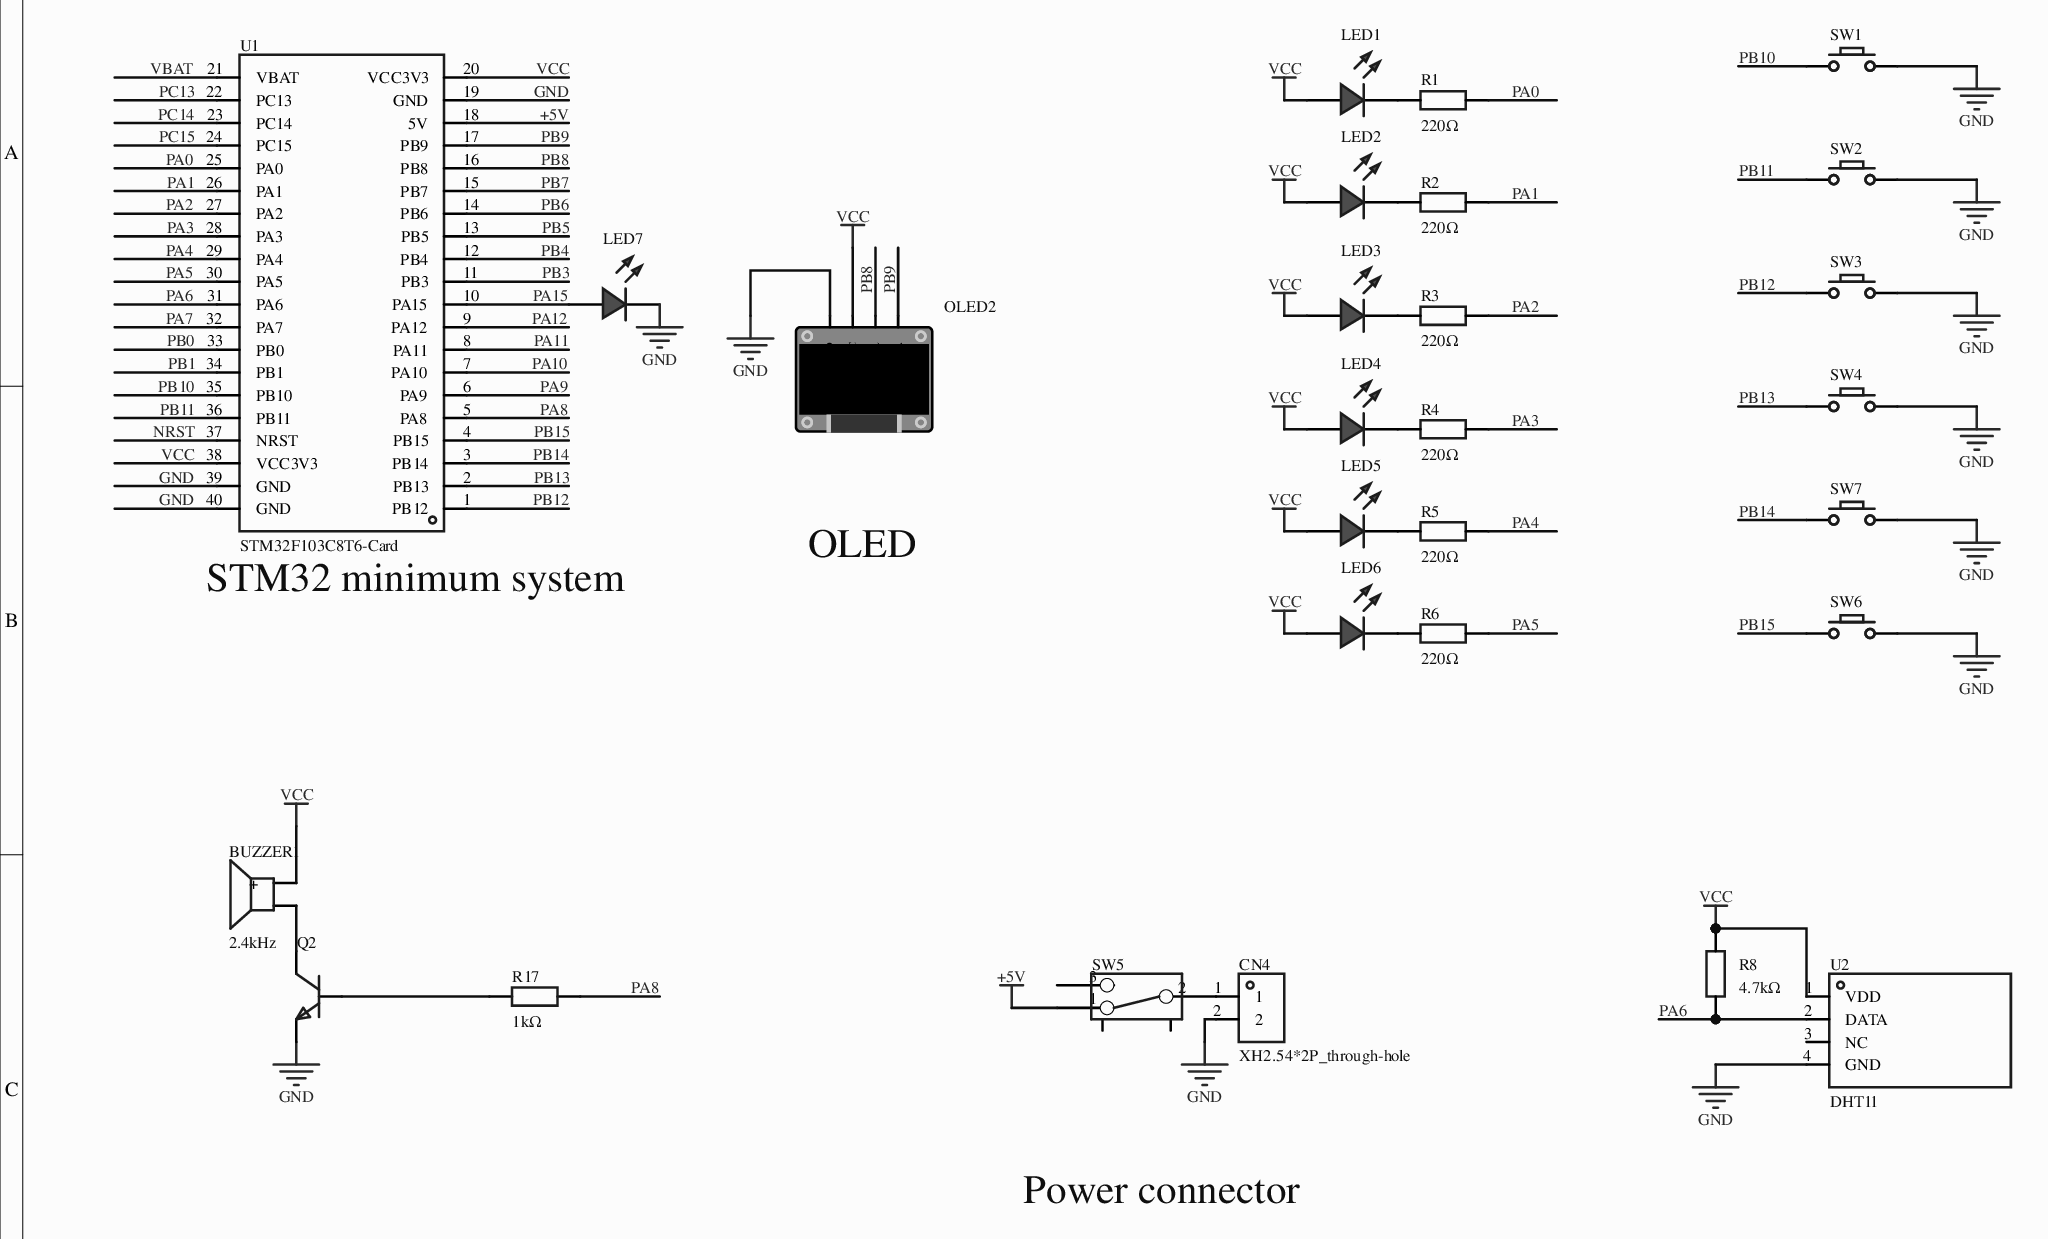
[diagram p0: MISC51258-3.schdoc]
# Altium project MISC51258-2.PrjPcb
1 sheet, 28 parts. Net scope: global (net labels, ports and power ports of the same name join across sheets).
Board file: MISC51258.pcbdoc

## Sheet MISC51258-3.schdoc
size 297 x 209 mm; Version: V1.0; @Project Name: MISC51258; @Page Count: 1; @Update Date: 2026-05-12; @Create Date: 2026-05-12; @Schematic Name: MISC51258; @Page No: 1; @Create Time: 23:22:16; @Update Time: 17:32:40; @Board Name: MISC51258

### Parts
BUZZER1  2.4kHz  [BUZ-TH_BD12.0-P7.60-D0.6-FD]
CN4  XH2.54*2P_through-hole  [CONN-TH_2P-P2.50-XH2.54-2P]
LED1  (no value)  [LED_TH-3mm]
LED2  (no value)  [LED_TH-3mm]
LED3  (no value)  [LED_TH-3mm]
LED4  (no value)  [LED_TH-3mm]
LED5  (no value)  [LED_TH-3mm]
LED6  (no value)  [LED_TH-3mm]
LED7  (no value)  [LED_TH-3mm]
OLED2  (no value)  [0.96OLED_4P]
Q2  (no value)  [S8050_TO_92]
R1  220Ω  [Res_1/8W]
R2  220Ω  [Res_1/8W]
R3  220Ω  [Res_1/8W]
R4  220Ω  [Res_1/8W]
R5  220Ω  [Res_1/8W]
R6  220Ω  [Res_1/8W]
R8  4.7kΩ  [Res_1/8W]
R17  1kΩ  [R0603]
SW1  (no value)  [Key_TH_3.5x6x4.3]
SW2  (no value)  [Key_TH_3.5x6x4.3]
SW3  (no value)  [Key_TH_3.5x6x4.3]
SW4  (no value)  [Key_TH_3.5x6x4.3]
SW5  (no value)  [拨动开关]
SW6  (no value)  [Key_TH_3.5x6x4.3]
SW7  (no value)  [Key_TH_3.5x6x4.3]
U1  STM32F103C8T6-Card  [CONN-TH_L53.3-W22.9_STM32F103C8T6-CARD]
U2  DHT11  [SENSOR-TH_DHT11]

### Nets
+5V: SW5.1 U1.18(5V)
GND: CN4.2 LED7.2(A) OLED2.1(GND) Q2.1(E) SW1.B SW2.B SW3.B SW4.B SW6.B SW7.B U1.19(GND) U1.39(GND) U1.40(GND) U2.4(GND)
VCC: BUZZER1.1(+) LED1.1(C) LED2.1(C) LED3.1(C) LED4.1(C) LED5.1(C) LED6.1(C) OLED2.2(VCC) R8.2 U1.20(VCC3V3) U1.38(VCC3V3) U2.1(VDD)
NRST: U1.37(NRST)
PA0: R1.2 U1.25(PA0)
PA1: R2.2 U1.26(PA1)
PA2: R3.2 U1.27(PA2)
PA3: R4.2 U1.28(PA3)
PA4: R5.2 U1.29(PA4)
PA5: R6.2 U1.30(PA5)
PA6: R8.1 U1.31(PA6) U2.2(DATA)
PA7: U1.32(PA7)
PA8: R17.1 U1.5(PA8)
PA9: U1.6(PA9)
PA10: U1.7(PA10)
PA11: U1.8(PA11)
PA12: U1.9(PA12)
PA15: LED7.1(C) U1.10(PA15)
PB0: U1.33(PB0)
PB1: U1.34(PB1)
PB3: U1.11(PB3)
PB4: U1.12(PB4)
PB5: U1.13(PB5)
PB6: U1.14(PB6)
PB7: U1.15(PB7)
PB8: OLED2.3(SCL) U1.16(PB8)
PB9: OLED2.4(SDA) U1.17(PB9)
PB10: SW1.A U1.35(PB10)
PB11: SW2.A U1.36(PB11)
PB12: SW3.A U1.1(PB12)
PB13: SW4.A U1.2(PB13)
PB14: SW7.A U1.3(PB14)
PB15: SW6.A U1.4(PB15)
PC13: U1.22(PC13)
PC14: U1.23(PC14)
PC15: U1.24(PC15)
VBAT: U1.21(VBAT)
NetBUZZER1_2: BUZZER1.2 Q2.3(C)
NetCN4_1: CN4.1 SW5.2
NetLED1_2: LED1.2(A) R1.1
NetLED2_2: LED2.2(A) R2.1
NetLED3_2: LED3.2(A) R3.1
NetLED4_2: LED4.2(A) R4.1
NetLED5_2: LED5.2(A) R5.1
NetLED6_2: LED6.2(A) R6.1
NetQ2_2: Q2.2(B) R17.2

Not connected (* = marked no-connect by the designer): SW5 3 4 5; U2 3(NC)

### Notes on the sheet
- (near U1) STM32 minimum system
- OLED
- Power connector

### Library data of the parts
BUZZER1 = TMB12A05_C96093: Driver mode: active (built-in driver circuit); construction type: electromagnetic; rated voltage: -; frequency: 2.4kHz; sound pressure (SPL): 85dB;; Manufacturer: 华能; 3D Model: 16ab50e14c5b4f2c986c135bdba60e37; 3D Model Transform: 472.44,472.176,0,90,0,0,-0.787,0,-177.165; Voltage - Supply: 4V~8V; AddInBom: yes; ModelName: BUZ-TH_D12.0-H9.5-P7.60; Symbol: TMB12A05; Device: TMB12A05_C96093; LCSC Part Name: TMB12A05; Supplier Part: C96093; Manufacturer Part: TMB12A05; Supplier Footprint: 插件,D=12mm; JLCPCB Part Class: Extended library; Datasheet: https://atta.szlcsc.com/upload/public/pdf/source/20241025/8A17FE04D767D19A35A06DEF9A82AB1E.pdf; Supplier: LCSC; Driver Circuitry: Active (built-in driver circuit); Technology: Electromagnetic; Voltage Rating: -; Value: 2.4kHz; Current Consumption: -; Sound Pressure Level(SPL): 85dB; Diameter(φD): 12mm; Length: -; Width: -; Height: 9.8mm; Operating Temperature: -; ConvertToPcb: yes; FootprintName: BUZ-TH_BD12.0-P7.60-D0.6-FD
CN4 = XH2.54*2P_直插: 3D Model: 325c595e30db4df8abe76612dd40b0fa0819f05c4eef4c71ace90d822a990e87; 3D Model Transform: 295.275,228.346,0,180,0,0,-0.002,-20.079,-137.795; AddInBom: yes; Device: XH2.54*2P_through-hole; Symbol: XH2.54*2P_through-hole; LCSC Part Name: XH2.54*2P_直插; Supplier Part: C9900008615; Manufacturer Part: XH2.54*2P_直插; Supplier Footprint: XH2.54_2P; JLCPCB Part Class: Extended Part; Supplier: LCSC; FootprintName: CONN-TH_2P-P2.50-XH2.54-2P; ConvertToPcb: yes; ModelName: CONN-TH_2P-P2.50-XH2.54-2P
LED1 = LED_TH-R_3mm: ConvertToPcb: yes; ModelId: a497c992633541038a38947cdc58012f0819f05c4eef4c71ace90d822a990e87; ModelName: LED-TH-3mm_R; ModelTransform: 141.274,153.327,0,0,0,0,-5.984,0,-137.795; Symbol: LED_TH-R; Device: LED_TH-R_3mm; AddInBom: yes; FootprintName: LED_TH-3mm; Supplier Footprint: 插件
LED2-LED7 = LED_TH-R_3mm: 3D Model: a497c992633541038a38947cdc58012f0819f05c4eef4c71ace90d822a990e87; 3D Model Transform: 141.274,153.327,0,0,0,0,-5.984,0,-137.795; ConvertToPcb: yes; ModelName: LED-TH-3mm_R; Symbol: LED_TH-R; Device: LED_TH-R_3mm; Supplier Footprint: 插件; AddInBom: yes; FootprintName: LED_TH-3mm
OLED2 = 0.96OLED模块_4P: Symbol: 0.96OLED module_4P; 3D Model: 79c000fdb68d45a296c2e9bedf4f9055; 3D Model Transform: 1393.69792,1318.895,0,0,0,0,0,-560.079,-137.795; ConvertToPcb: yes; Device: 0.96OLED module_4P; Supplier Footprint: 插件; AddInBom: yes; FootprintName: 0.96OLED_4P; ModelName: 0.96OLED_4P
Q2 = S8050_TO_NPN: ConvertToPcb: yes; ModelId: aafe8e06f2154e7c93506efd0d6632dd; ModelName: TO-92-3_L4.9-W3.7-P1.27-L; ModelTransform: 180.78,141.44,417.3,0,0,0,0,0,-200; Symbol: S8050_TO_NPN; Device: S8050_TO_NPN; AddInBom: yes; Supplier Footprint: TO-92; FootprintName: S8050_TO_92
R1-R6 R8 = Res_AXIAL-1/8W: Symbol: Resistor; 3D Model: b2b5ae7ae4c642178fe0039925c86a3f0819f05c4eef4c71ace90d822a990e87; 3D Model Transform: 282.86,66.88,253.09,0,0,0,0,0,-191; ConvertToPcb: yes; ModelName: RES-TH_BD1.8-L3.2-P7.20-D0.4; Device: Res_AXIAL-1/8W; Supplier Footprint: 轴向引线; AddInBom: yes; FootprintName: Res_1/8W
  R1-R6: Value: 220Ω
  R8: Value: 4.7kΩ
R17 = RC0603FR-071KL: Thick film resistor; resistance: 1kΩ; tolerance: ±1%; power: 100mW; working voltage: 75V; temperature coefficient: ±100ppm/℃;; Manufacturer: YAGEO(国巨); 3D Model: fc143cca1e79419f9cd78b61e9279f08; 3D Model Transform: 31.8897,63.7794,0,90,0,0,0,0,0; AddInBom: yes; Symbol: RC0603FR-071KL; Device: RC0603FR-071KL; LCSC Part Name: 厚膜电阻 1kΩ ±1% 100mW; Supplier Part: C22548; Manufacturer Part: RC0603FR-071KL; Supplier Footprint: 0603; JLCPCB Part Class: Extended library; Datasheet: https://atta.szlcsc.com/upload/public/pdf/source/20180316/70C0E2BDAE7FCC62C531A5A58D202EE1.pdf; Supplier: LCSC; Type: Thick film resistor; Value: 1kΩ; Tolerance: ±1%; Power(Watts): 100mW; Voltage-Supply(Max): 75V; Temperature Coefficient: ±100ppm/℃; Operating Temperature: -55℃~+155℃; Overload Voltage (Max): 75V; Operating Temperature Range: -55℃~+155℃; ConvertToPcb: yes; FootprintName: R0603; ModelName: R0603
SW1-SW4 SW6 SW7 = Key_TH_3.5x6x4.3: ConvertToPcb: yes; ModelId: c3523f9014d949d7ba5445190a3178990819f05c4eef4c71ace90d822a990e87; ModelName: SW-TH_L6.0-W3.5-H5.0-P6.5; ModelTransform: 308.49,137.8,335.08,0,0,0,0,0,-129.92; Symbol: Key_TH_3.5x6x4.3; Device: Key_TH_3.5x6x4.3; AddInBom: yes; Supplier Footprint: 插件; FootprintName: Key_TH_3.5x6x4.3
SW5 = 拨动开关_正: Device: Toggle switch_positive; Symbol: Toggle switch; 3D Model: 4321fe59a4074cbfb4989553f297c68f0819f05c4eef4c71ace90d822a990e87; 3D Model Transform: 370.09,208.7,472.35,0,0,0,0,0,-110; ConvertToPcb: yes; ModelName: SW-TH_SS-12D02-VG4; Supplier Footprint: 插件; FootprintName: Toggle switch; AddInBom: yes
U1 = STM32F103C8T6-Card: AddInBom: yes; Device: STM32F103C8T6-Card; Symbol: STM32F103C8T6-CARD; FootprintName: CONN-TH_L53.3-W22.9_STM32F103C8T6-CARD; LCSC Part Name: STM32F103C8T6-Card; SupplierPart: C9900077949; ManufacturerPart: STM32F103C8T6-Card; Supplier Footprint: 插件; Supplier: LCSC; ConvertToPcb: yes
U2 = DHT11: New capacitive digital temperature and humidity sensor; old model discontinued; 16.1x12.6x5.8mm; Manufacturer: 广州奥松; AddInBom: yes; ModelId: 6dde47d4d8bf4fa598dffcc067449c1d; ModelTransform: 236.25937,492.125,0,270,0,0,0,-11.811,-196.85; Symbol: DHT11; Device: DHT11; LCSC Part Name: 新款电容式数字温湿度传感器,老款已停产16.1x12.6x5.8mm DHT11  电容式传感器; SupplierPart: C117051; ManufacturerPart: DHT11; Supplier Footprint: SIP-4; JLCPCB Part Class: Extended library; Datasheet: https://atta.szlcsc.com/upload/public/pdf/source/20170703/1499081238365.pdf; Supplier: LCSC; ConvertToPcb: yes; FootprintName: SENSOR-TH_DHT11; ModelName: SENSOR-TH_DHT11